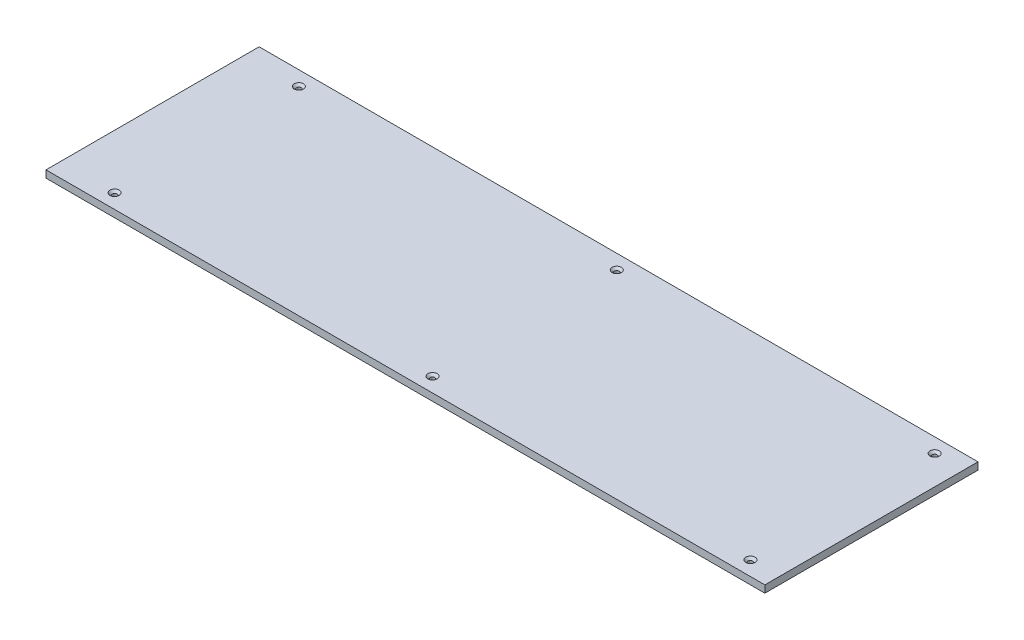
SolidWorks part; units mm, degrees
material "PE"
ref_plane "Front Plane" through (0, 0, 0) normal (0, 0, 1) x (1, 0, 0)
ref_plane "Top Plane" through (0, 0, 0) normal (0, 1, 0) x (1, 0, 0)
ref_plane "Right Plane" through (0, 0, 0) normal (1, 0, 0) x (0, 0, -1)
sketch "Sketch1" plane through (0, 0, 0) normal (0, 1, 0) x (1, 0, 0)
  line L1 (0, 0) -> (995, 0)
  line L2 (0, 0) -> (0, -295)
  line L3 (0, -295) -> (995, -295)
  line L4 (995, 0) -> (995, -295)
  dimension "D1" = 995
  dimension "D2" = 295
extrude "Boss-Extrude1" add sketch "Sketch1" along normal blind 10
hole_wizard "Hole Size (% based) Hexalobular Socket Semi-Countersunk Screw Type1" positions "Sketch2" profile "Sketch3" countersink size "M6" standard "GB"
sketch "Sketch2" plane through (0, 10, 0) normal (0, 1, 0) x (1, 0, 0)
  line L0 (515, 0) -> (515, -20) construction
  line L3 (0, -147.5) -> (120.9859, -147.5) construction
  line L4 (0, 0) -> (0, -295) construction
  line L5 (995, -295) -> (995, 0) construction
  point P0 (75, -20)
  point P2 (75, -275)
  point P4 (515, -20)
  point P6 (515, -275)
  point P20 (955, -275)
  point P21 (955, -20)
  dimension "D1" = 880
  dimension "D2" = 255
  dimension "D3" = 40
sketch "Sketch3" plane through (75, 10, 20) normal (1, 0, 0) x (0, 0, 1)
  line L0 (0, 0) -> (0, 21.7328)
  line L1 (0, 21.7328) -> (3.3, 19.75)
  line L2 (3.3, 19.75) -> (3.3, 3.1)
  line L3 (3.3, 3.1) -> (6.4, 0)
  line L5 (6.4, 0) -> (0, 0)
  line L6 (-3.3, 3.1) -> (-6.4, 0) construction
  line L10 (0, 21.7328) -> (-3.3, 19.75) construction
  line L11 (0, -6.35) -> (0, 107.95) construction
  dimension "孔直径" = 6.6
  dimension "孔深度" = 19.75
  dimension "近端锥形沉头孔直径" = 12.8
  dimension "近端锥形沉头孔角度" = 90
  dimension "导头角度" = 118
